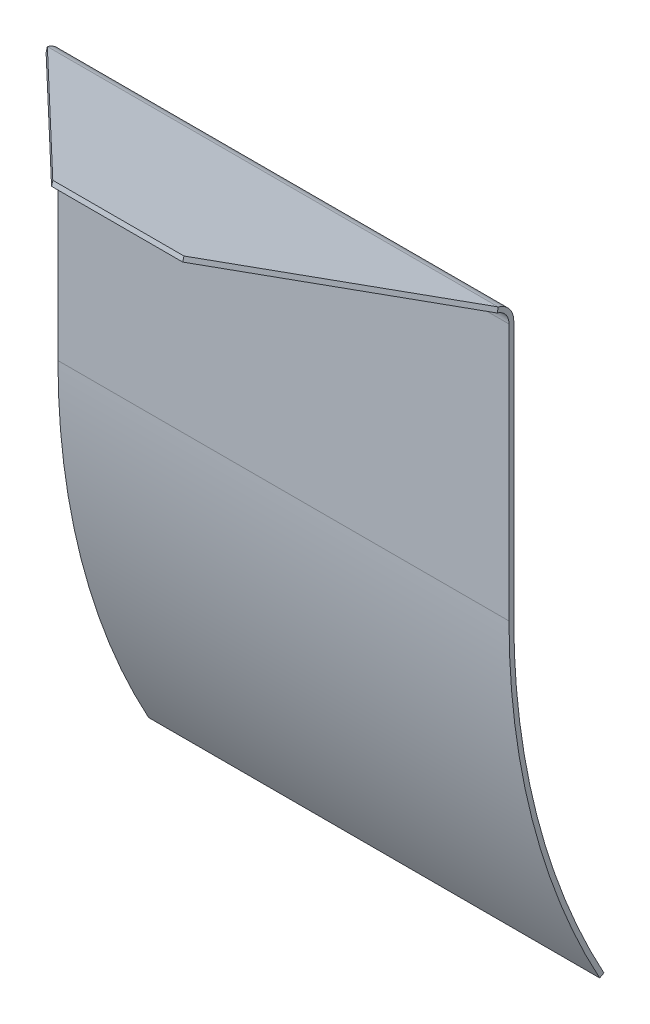
SolidWorks part; units mm, degrees
ref_plane "Front Plane" through (0, 0, 0) normal (0, 0, 1) x (1, 0, 0)
ref_plane "Top Plane" through (0, 0, 0) normal (0, 1, 0) x (1, 0, 0)
ref_plane "Right Plane" through (0, 0, 0) normal (1, 0, 0) x (0, 0, -1)
sketch "Sketch1" plane through (0, 0, 0) normal (1, 0, 0) x (0, 0, -1)
  line L1 (-201.1296, -110.1152) -> (-202.4453, -110.8356)
  line L2 (0, 0) -> (-201.1296, -110.1152) construction
  line L3 (0, 0) -> (-229.3, 0) construction
  line L4 (-229.3, 0) -> (-229.3, 80.4)
  line L6 (-234.1177, 86.6785) -> (-282.414, 99.6195)
  line L7 (-282.414, 99.6195) -> (-282.8022, 98.1706)
  line L9 (-230.8, 1.5) -> (-230.8, 1.5)
  line L10 (-230.8, 80.4) -> (-230.8, 0)
  line L11 (-282.8022, 98.1706) -> (-234.5059, 85.2296)
  line L12 (-281.3533, 97.7824) -> (-281.3533, 97.7824)
  line L13 (-230.8, 1.5) -> (-230.8, 80.4) construction
  line L14 (-234.5059, 85.2296) -> (-281.3533, 97.7824) construction
  arc A0 (-229.3, 0) -> (-201.1296, -110.1152) centre (0, 0) ccw
  arc A1 (-230.8, 0) -> (-202.4453, -110.8356) centre (0, 0) ccw
  arc A2 (-229.3, 80.4) -> (-234.1177, 86.6785) centre (-235.8, 80.4) ccw
  circle A3 centre (0, 0) radius 229.3 construction
  circle A4 centre (0, 0) radius 230.8 construction
  arc A5 (-230.8, 1.5) -> (-230.8, 1.5) centre (-230.8, 1.5) ccw
  arc A6 (-230.8, 1.5) -> (-230.8, 1.5) centre (-230.8, 1.5) cw
  arc A7 (-230.8, 80.4) -> (-234.5059, 85.2296) centre (-235.8, 80.4) ccw
  point P1 (230.8, 0)
  point P4 (219.2807, 67.0408)
  dimension "D1" = 458.6
  dimension "D6" = 6.5
  dimension "D2" = 1.5
  dimension "D3" = 28.7
  dimension "D4" = 1.5
  dimension "D5" = 75
  dimension "D8" = 80.4
  dimension "D9" = 50
  dimension "D7" = 1.5
extrude "Boss-Extrude1" add sketch "Sketch1" along normal mid plane 141 contours A7 L10 A1 L1 A0 L4 A2 L6 L7 L11
chamfer "Chamfer1" distance 50 angle 45 2 edges at (-70.5, 98.895, 282.6081) (70.5, 98.895, 282.6081)
